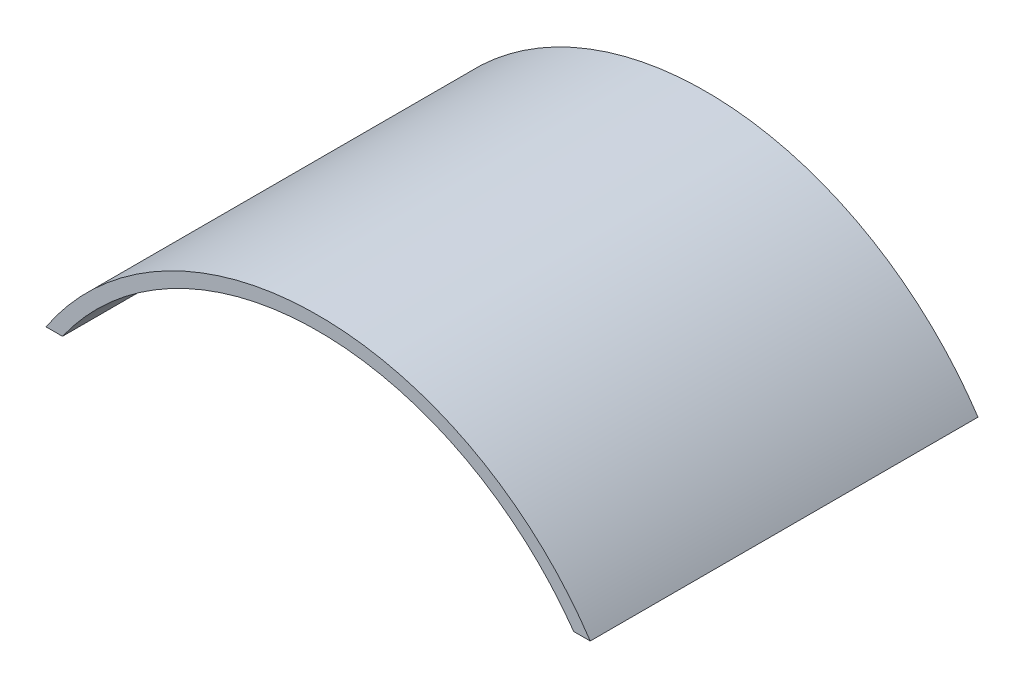
SolidWorks part; units mm, degrees
material "橡胶"
ref_plane "Front Plane" through (0, 0, 0) normal (0, 0, 1) x (1, 0, 0)
ref_plane "Top Plane" through (0, 0, 0) normal (0, 1, 0) x (1, 0, 0)
ref_plane "Right Plane" through (0, 0, 0) normal (1, 0, 0) x (0, 0, -1)
sketch "Sketch1" plane through (0, 0, 0) normal (0, 0, 1) x (1, 0, 0)
  line L0 (0, 0) -> (0, 48) construction
  line L1 (-40, 26.533) -> (-37.5766, 26.533)
  line L2 (37.5766, 26.533) -> (40, 26.533)
  arc A0 (40, 26.533) -> (-40, 26.533) centre (0, 0) ccw
  arc A1 (37.5766, 26.533) -> (-37.5766, 26.533) centre (0, 0) ccw
  arc A3 (38.3333, 25.4275) -> (-38.3333, 25.4275) centre (0, 0) ccw construction
  dimension "D1" = 96
  dimension "D2" = 80
  dimension "D3" = 2
extrude "Boss-Extrude1" add sketch "Sketch1" along normal mid plane 57
